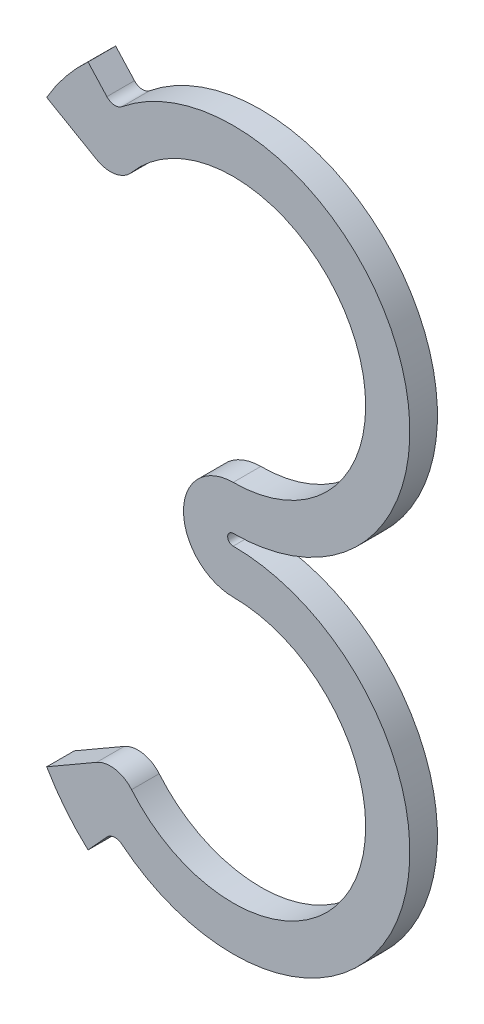
SolidWorks part; units mm, degrees
ref_plane "前视基准面" through (0, 0, 0) normal (0, 0, 1) x (1, 0, 0)
ref_plane "上视基准面" through (0, 0, 0) normal (0, 1, 0) x (1, 0, 0)
ref_plane "右视基准面" through (0, 0, 0) normal (1, 0, 0) x (0, 0, -1)
sketch "草图2" plane through (0, 0, 0) normal (0, 0, 1) x (1, 0, 0)
  line L0 (-9.6076, 9.9209) -> (7.5886, 9.9209) construction
  line L1 (-12.3924, -6.5791) -> (11, -6.5791) construction
  line L2 (0, 15.4905) -> (0, -17.231) construction
  line L4 (-4.5, -6.5791) -> (-0.5, -6.5791)
  line L5 (-10.3923, 15.9209) -> (-16.8875, 19.6709)
  line L6 (-10.7847, 21.7399) -> (-13.1439, 24.3254)
  arc A0 (0, -6.0791) -> (-0.5, -6.5791) centre (0, -6.5791) ccw
  arc A1 (0, -2.0791) -> (-4.5, -6.5791) centre (0, -6.5791) ccw
  arc A2 (0, -2.0791) -> (-10.3923, 15.9209) centre (0, 9.9209) ccw
  arc A3 (0, -6.0791) -> (-10.7847, 21.7399) centre (0, 9.9209) ccw
  arc A4 (-13.1439, 24.3254) -> (-16.8875, 19.6709) centre (0, 9.9209) ccw
  point P13 (-0.3536, -6.2256)
  dimension "D2" = 0.5
  dimension "D3" = 4.5
  dimension "D4" = 12
  dimension "D5" = 4
  dimension "D1" = 16.5
  dimension "D6" = 60
ref_plane "基准面1" through (0, -6.5791, 0) normal (0, 1, 0) x (1, 0, 0)
extrude "凸台-拉伸1" add sketch "草图2" along normal blind 2.5
fillet "圆角1" radius 1 1 edges at (-10.7847, 21.7399, 1.25)
fillet "圆角2" radius 2.5 1 edges at (-10.3923, 15.9209, 1.25)
mirror "镜向1" about plane through (0, -6.5791, 0) normal (0, 1, 0) of "圆角2", "圆角1", "凸台-拉伸1"
